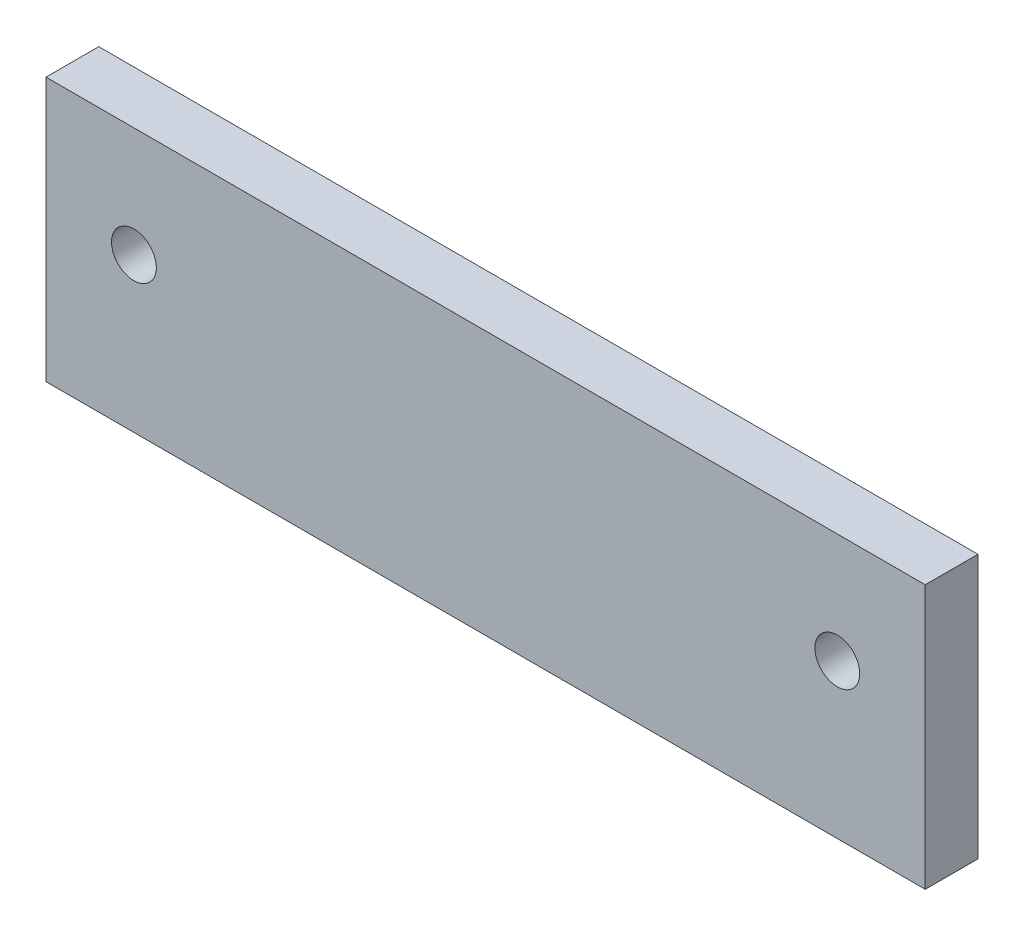
SolidWorks part; units mm, degrees
material "1023 碳钢板 (SS)"
ref_plane "Front Plane" through (0, 0, 0) normal (0, 0, 1) x (1, 0, 0)
ref_plane "Top Plane" through (0, 0, 0) normal (0, 1, 0) x (1, 0, 0)
ref_plane "Right Plane" through (0, 0, 0) normal (1, 0, 0) x (0, 0, -1)
sketch "Sketch1" plane through (0, 0, 0) normal (0, 0, 1) x (1, 0, 0)
  line L1 (100, 30) -> (-100, 30)
  line L2 (100, 30) -> (100, -30)
  line L3 (100, -30) -> (-100, -30)
  line L4 (-100, 30) -> (-100, -30)
  line L5 (100, 30) -> (-100, -30) construction
  line L6 (100, -30) -> (-100, 30) construction
  point P0 (0, 0)
  dimension "D1" = 200
  dimension "D2" = 60
extrude "Boss-Extrude1" add sketch "Sketch1" along normal blind 12 contours L2 L1 L4 L3
sketch "Sketch2" plane through (0, 0, 12) normal (0, 0, 1) x (1, 0, 0)
  line L0 (100, 30) -> (-100, 30) construction
  circle A0 centre (-80, 5) radius 4.5
  circle A1 centre (80, 5) radius 4.5
  dimension "D3" = 25
  dimension "D4" = 9
  dimension "D1" = 160
  dimension "D2" = 80
hole_wizard "M12 Tapped Hole1" positions "Sketch3" profile "Sketch4" tap size "M12" standard "ISO"
sketch "Sketch3" plane through (0, 0, 12) normal (0, 0, 1) x (1, 0, 0)
  point P0 (-80, 5)
  point P3 (80, 5)
sketch "Sketch4" plane through (-80, 5, 12) normal (1, 0, 0) x (0, -1, 0)
  line L0 (0, 0) -> (0, 32.3144)
  line L1 (0, 32.3144) -> (5.1, 29.25)
  line L2 (5.1, 29.25) -> (5.1, 0)
  line L5 (5.1, 0) -> (0, 0)
  line L10 (0, 32.3144) -> (-5.1, 29.25) construction
  line L11 (0, -6.35) -> (0, 107.95) construction
  dimension "螺纹孔钻头直径" = 10.2
  dimension "螺纹孔钻头深度" = 29.25
  dimension "导头角度" = 118
cosmetic thread "Hole Thread Line 1" parameters "D1"=24, "D2"=12
cosmetic thread "Hole Thread Line 2" parameters "D1"=24, "D2"=12
